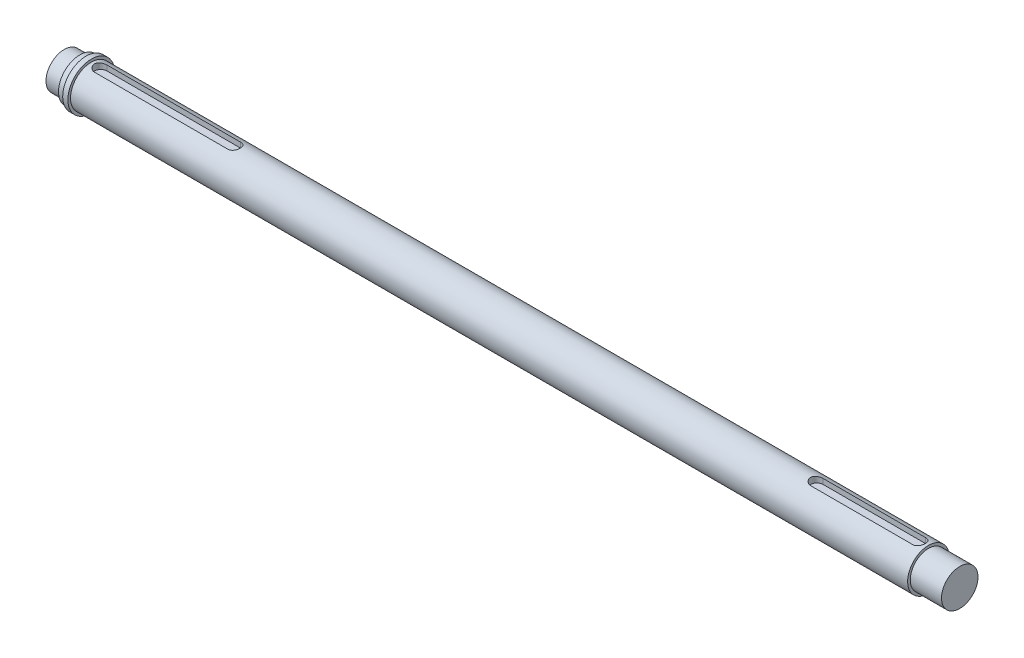
from build123d import *

# Parameters (mm, degrees)
SKETCH_1_R          = 20
EXTRUDE_1_DEPTH     = 803
SKETCH_2_R          = 17.5
EXTRUDE_2_DEPTH     = 30
SKETCH_3_R          = 22.5
EXTRUDE_3_DEPTH     = 5
SKETCH_4_R          = 20.5
EXTRUDE_4_DEPTH     = 6
EXTRUDE_START       = 15
SKETCH_5_R          = 17.5
EXTRUDE_5_DEPTH     = 15
CUT_EXTRUDE_1_DEPTH = 5.92


with BuildPart() as part:
    # 草图1 → 凸台-拉伸1 (new body)
    with BuildSketch(Plane(origin=(0, 0, 0), x_dir=(0, 0, -1), z_dir=(1, 0, 0))):
        Circle(SKETCH_1_R)
    extrude(amount=EXTRUDE_1_DEPTH)

    # 草图2 → 凸台-拉伸2 (add)
    with BuildSketch(Plane(origin=(803, 0, 0), x_dir=(0, 0, -1), z_dir=(1, 0, 0))):
        Circle(SKETCH_2_R)
    extrude(amount=EXTRUDE_2_DEPTH)

    # 草图3 → 凸台-拉伸3 (add)
    with BuildSketch(Plane.ZY):
        Circle(SKETCH_3_R)
    extrude(amount=EXTRUDE_3_DEPTH)

    # 草图4 → 凸台-拉伸4 (add)
    with BuildSketch(Plane.ZY.offset(5)):
        Circle(SKETCH_4_R)
    extrude(amount=EXTRUDE_4_DEPTH)

    # 草图5 → 凸台-拉伸5 (add)
    with BuildSketch(Plane.ZY.offset(11).offset(EXTRUDE_START)):
        with Locations(Location((0, 0, 0), (0, 0, 180))):
            Circle(SKETCH_5_R)
    extrude(amount=-EXTRUDE_5_DEPTH)

    # 草图6 → 切除-拉伸1 (cut)
    with BuildSketch(Plane(origin=(0, 20, 0), x_dir=(1, 0, 0), z_dir=(0, 1, 0))):
        with BuildLine():
            Line((9, 6), (137, 6))
            ThreePointArc((137, 6), (143, 0), (137, -6))
            Line((137, -6), (9, -6))
            ThreePointArc((9, -6), (3, 0), (9, 6))
        make_face()
        with BuildLine():
            Line((794, -6), (696, -6))
            ThreePointArc((696, -6), (690, 0), (696, 6))
            Line((696, 6), (794, 6))
            ThreePointArc((794, 6), (800, 0), (794, -6))
        make_face()
    extrude(amount=-CUT_EXTRUDE_1_DEPTH, mode=Mode.SUBTRACT)


solid = part.part
